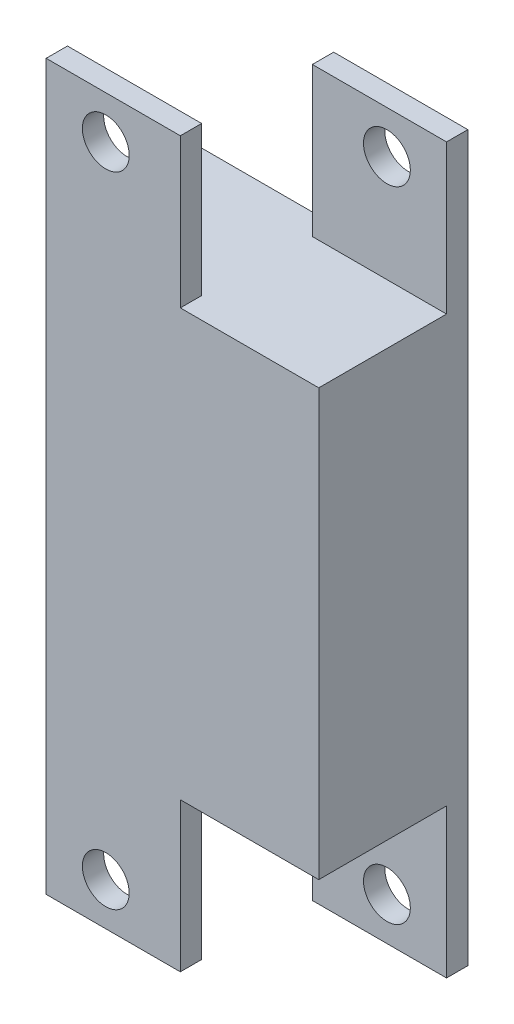
SolidWorks part; units mm, degrees
material "Q235A"
ref_plane "前视基准面" through (0, 0, 0) normal (0, 0, 1) x (1, 0, 0)
ref_plane "上视基准面" through (0, 0, 0) normal (0, 1, 0) x (1, 0, 0)
ref_plane "右视基准面" through (0, 0, 0) normal (1, 0, 0) x (0, 0, -1)
sketch "草图1" plane through (0, 0, 0) normal (0, 0, 1) x (1, 0, 0)
  line L1 (-32, 85) -> (32, 85)
  line L2 (-32, 85) -> (-32, -85)
  line L3 (-32, -85) -> (32, -85)
  line L4 (32, 85) -> (32, -85)
  line L5 (-32, 85) -> (32, -85) construction
  line L6 (-32, -85) -> (32, 85) construction
  point P0 (0, 0)
  dimension "D1" = 64
  dimension "D2" = 170
extrude "凸台-拉伸1" add sketch "草图1" along normal blind 35
sketch "草图3" plane through (0, 0, 35) normal (0, 0, 1) x (1, 0, 0)
  line L0 (-32, 85) -> (-32, -85) construction
  line L1 (32, 85) -> (-0.5, 85)
  line L2 (32, 85) -> (32, 50)
  line L3 (32, 50) -> (-0.5, 50)
  line L4 (-0.5, 85) -> (-0.5, 50)
  line L5 (32, -85) -> (-0.5, -85)
  line L6 (32, -85) -> (32, -50)
  line L7 (32, -50) -> (-0.5, -50)
  line L8 (-0.5, -85) -> (-0.5, -50)
  dimension "D1" = 35
  dimension "D2" = 35
  dimension "D3" = 31.5
extrude "切除-拉伸1" cut sketch "草图3" against normal blind 30
sketch "草图4" plane through (0, 0, 0) normal (0, 0, -1) x (-1, 0, 0)
  line L0 (-32, -85) -> (-32, 85) construction
  line L1 (32, 85) -> (-0.5, 85)
  line L2 (32, 85) -> (32, 50)
  line L3 (32, 50) -> (-0.5, 50)
  line L4 (-0.5, 85) -> (-0.5, 50)
  line L5 (32, -85) -> (-0.5, -85)
  line L6 (32, -85) -> (32, -50)
  line L7 (32, -50) -> (-0.5, -50)
  line L8 (-0.5, -85) -> (-0.5, -50)
  dimension "D1" = 31.5
  dimension "D2" = 35
  dimension "D3" = 35
extrude "切除-拉伸2" cut sketch "草图4" against normal blind 30
sketch "草图5" plane through (0, 0, 35) normal (0, 0, 1) x (1, 0, 0)
  line L0 (0, 0) -> (72.4281, 0) construction
  line L1 (-32, 85) -> (-32, -85) construction
  line L2 (32, 50) -> (32, 85) construction
  circle A0 centre (-18, 75) radius 5.5
  circle A1 centre (18, 75) radius 5.5
  circle A2 centre (18, -75) radius 5.5
  circle A3 centre (-18, -75) radius 5.5
  dimension "D1" = 14
  dimension "D2" = 14
  dimension "D3" = 75
  dimension "D4" = 11
  dimension "D5" = 11
extrude "切除-拉伸3" cut sketch "草图5" against normal through all both and the other way through all
